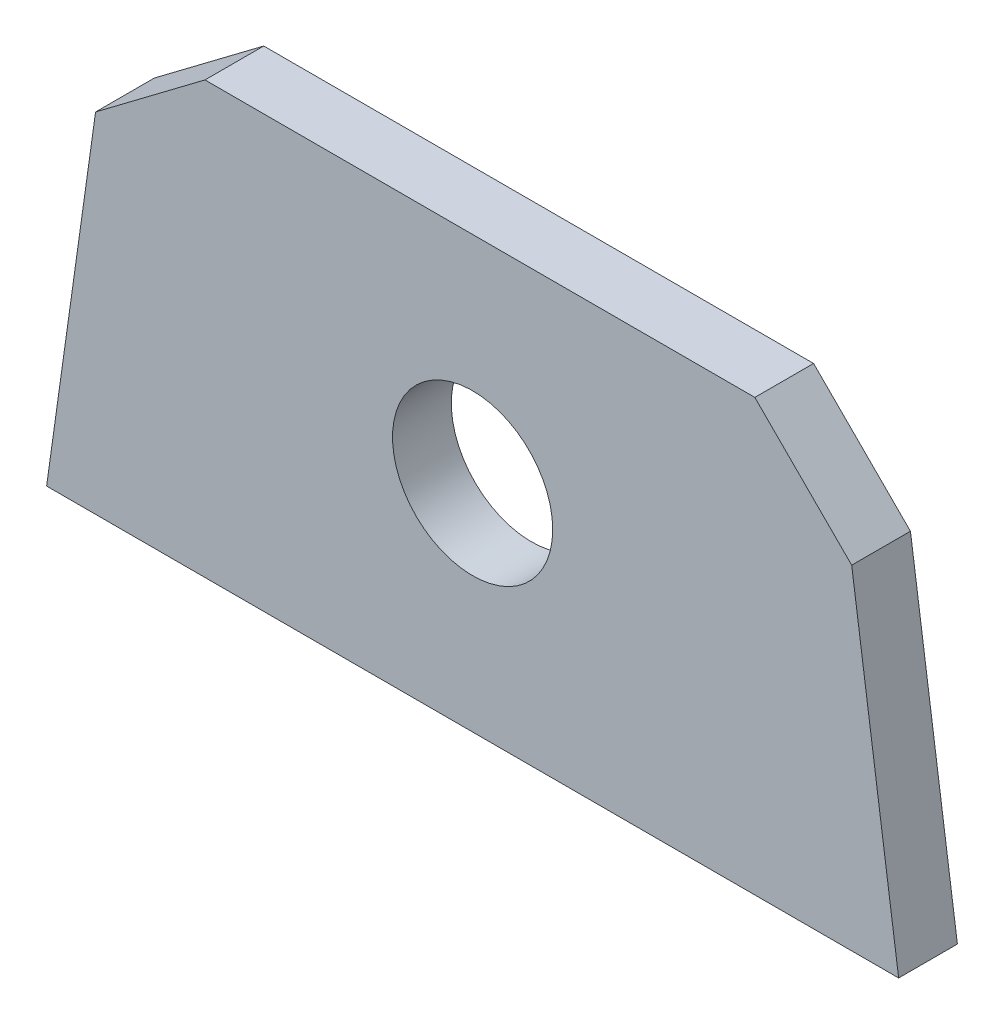
SolidWorks part; units mm, degrees
material "1023 碳钢板 (SS)"
ref_plane "前视基准面" through (0, 0, 0) normal (0, 0, 1) x (1, 0, 0)
ref_plane "上视基准面" through (0, 0, 0) normal (0, 1, 0) x (1, 0, 0)
ref_plane "右视基准面" through (0, 0, 0) normal (1, 0, 0) x (0, 0, -1)
sketch "草图1" plane through (0, 0, 0) normal (0, 0, 1) x (1, 0, 0)
  line L1 (43.5, 22) -> (-43.5, 22)
  line L2 (43.5, 22) -> (43.5, -22)
  line L3 (43.5, -22) -> (-43.5, -22)
  line L4 (-43.5, 22) -> (-43.5, -22)
  line L5 (43.5, 22) -> (-43.5, -22) construction
  line L6 (43.5, -22) -> (-43.5, 22) construction
  point P0 (0, 0)
  dimension "D1" = 87
  dimension "D2" = 44
extrude "凸台-拉伸1" add sketch "草图1" along normal blind 6
sketch "草图2" plane through (0, 0, 6) normal (0, 0, 1) x (1, 0, 0)
  line L0 (-43.5, -22) -> (43.5, -22) construction
  line L1 (-43.5, -22) -> (-37.3162, 22)
  line L2 (43.5, -22) -> (37.3162, 22)
  line L3 (43.5, 22) -> (-43.5, 22) construction
  line L4 (43.5, -22) -> (43.5, 22) construction
  line L5 (-43.5, 22) -> (-43.5, -22) construction
  line L6 (-43.5, 22) -> (-37.3162, 22)
  line L7 (-43.5, 22) -> (-43.5, -22)
  line L8 (37.3162, 22) -> (43.5, 22)
  line L9 (43.5, 22) -> (43.5, -22)
  circle A0 centre (0, 0) radius 8.1792
  dimension "D1" = 22
  dimension "D2" = 8
  dimension "D3" = 8
extrude "切除-拉伸1" cut sketch "草图2" against normal blind 6
chamfer "倒角1" distance 8.5 angle 45 2 edges at (37.3162, 22, 3) (-37.3162, 22, 3)
